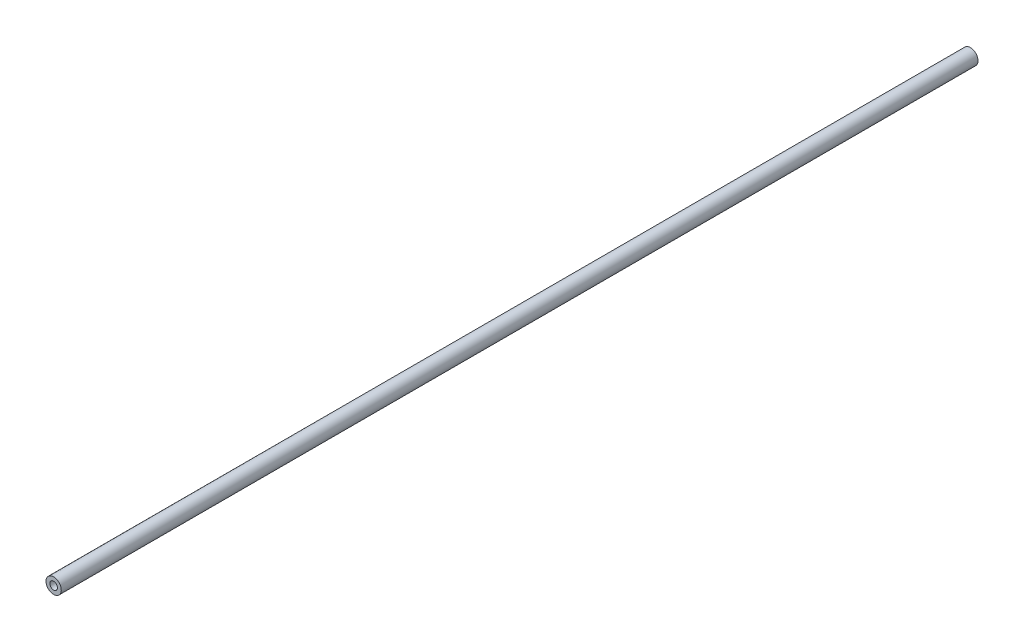
SolidWorks part; units mm, degrees
ref_plane "Front Plane" through (0, 0, 0) normal (0, 0, 1) x (1, 0, 0)
ref_plane "Top Plane" through (0, 0, 0) normal (0, 1, 0) x (1, 0, 0)
ref_plane "Right Plane" through (0, 0, 0) normal (1, 0, 0) x (0, 0, -1)
other "Configuration Table"
sketch "Sketch2" plane through (0, 0, 0) normal (0, 0, 1) x (1, 0, 0)
  circle A0 centre (0, 0) radius 2.5
  circle A1 centre (0, 0) radius 1.25
  dimension "D1" = 5
  dimension "D2" = 2.5
extrude "Boss-Extrude1" add sketch "Sketch2" along normal blind 300
ref_plane "Plane1" through (0, 2.5, 0) normal (0, 1, 0) x (1, 0, 0)
